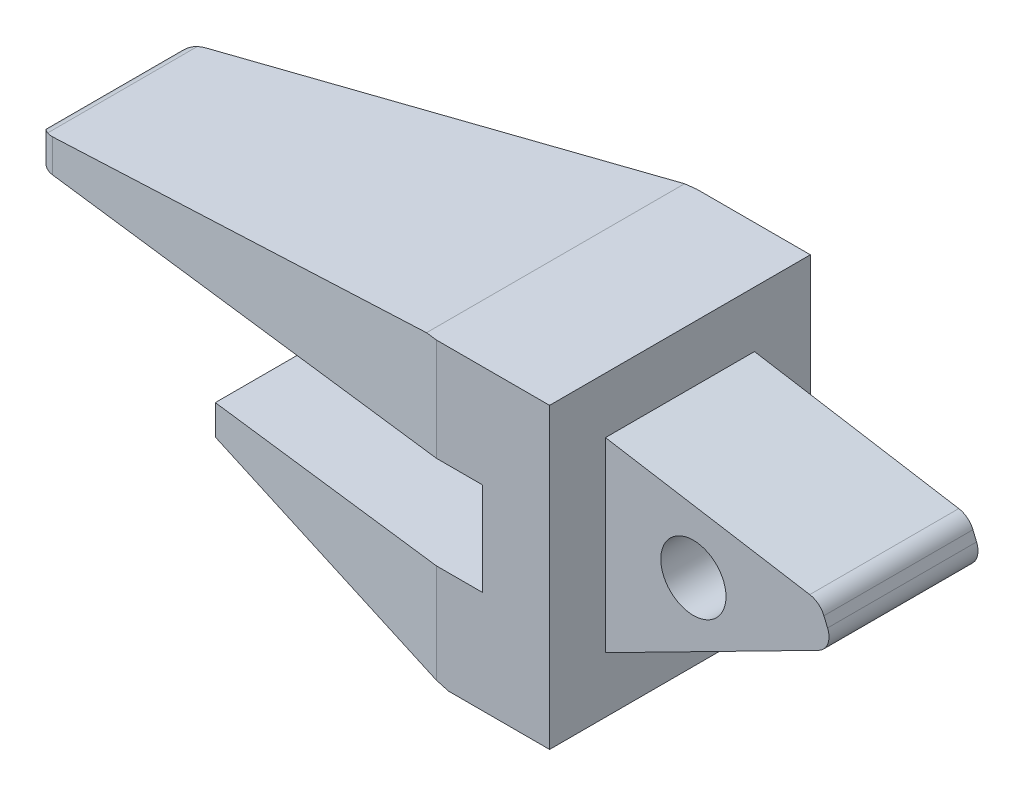
from build123d import *

# Parameters (mm, degrees)
BOSS_EXTRUDE1_DEPTH      = 80
CUT_EXTRUDE1_DEPTH       = 177.164695669
CUT_EXTRUDE1_DEPTH_BACK  = 177.164695669
SKETCH2_OUTSIDE_W        = 192.26
SKETCH2_OUTSIDE_H        = 119.26
BOSS_EXTRUDE2_DEPTH      = 20
BOSS_EXTRUDE2_DEPTH_BACK = 20
M20_TAPPED_HOLE1_D       = 17.5


with BuildPart() as part:
    # Sketch1 → Boss-Extrude1 (new body)
    with BuildSketch(Plane(origin=(0, 0, 0), x_dir=(1, 0, 0), z_dir=(0, 1, 0))):
        with BuildLine():
            Line((0, 14.689353522), (0, -14.689353522))
            ThreePointArc((0, -14.689353522), (1.507118597, -18.666037655), (5.271338899, -20.644943585))
            Line((5.271338899, -20.644943585), (122.6, -35))
            Line((122.6, -35), (153, -35))
            Line((153, -35), (153, 35))
            Line((153, 35), (122.6, 35))
            Line((122.6, 35), (5.271338899, 20.644943585))
            ThreePointArc((5.271338899, 20.644943585), (1.507118597, 18.666037655), (0, 14.689353522))
        make_face()
    extrude(amount=BOSS_EXTRUDE1_DEPTH)

    # Sketch2 outside → Cut-Extrude1 (cut, two sides: drawn at the far end of the back side and taken through both)
    with BuildSketch(Plane.XY.offset(-CUT_EXTRUDE1_DEPTH_BACK)):
        with Locations((76.5, 40)):
            Rectangle(SKETCH2_OUTSIDE_W, SKETCH2_OUTSIDE_H)
        with BuildLine():
            Line((153, 80), (153, 0))
            Line((153, 0), (125.9, 0))
            Line((125.9, 0), (55, 19.5))
            Line((55, 19.5), (55, 27.5))
            Line((55, 27.5), (135, 27.5))
            Line((135, 27.5), (135, 52.5))
            Line((135, 52.5), (0, 52.5))
            Line((0, 52.5), (0, 57.099356274))
            ThreePointArc((0, 57.099356274), (0.95248476, 59.69023467), (3.35632543, 61.047226972))
            Line((3.35632543, 61.047226972), (119.6, 80))
            Line((119.6, 80), (153, 80))
        make_face(mode=Mode.SUBTRACT)
    extrude(amount=CUT_EXTRUDE1_DEPTH + CUT_EXTRUDE1_DEPTH_BACK, mode=Mode.SUBTRACT)

    # Sketch3 → Boss-Extrude2 (add, two sides: drawn at the far end of the back side and taken through both)
    with BuildSketch(Plane.XY.offset(-BOSS_EXTRUDE2_DEPTH_BACK)):
        with BuildLine():
            Line((153, 65), (153, 15))
            Line((153, 15), (210.269952499, 44.180498289))
            ThreePointArc((210.269952499, 44.180498289), (212.69221031, 46.908347535), (212.616617933, 50.555645193))
            Line((212.616617933, 50.555645193), (211.637866551, 52.908901571))
            ThreePointArc((211.637866551, 52.908901571), (210.127565677, 54.906796263), (207.837878429, 55.921648096))
            Line((207.837878429, 55.921648096), (153, 65))
        make_face()
    extrude(amount=BOSS_EXTRUDE2_DEPTH + BOSS_EXTRUDE2_DEPTH_BACK)

    # M20 Tapped Hole1 (through all)
    with Locations(Plane.XY.offset(20)):
        with Locations((176.6, 44.2)):
            Hole(M20_TAPPED_HOLE1_D / 2)


solid = part.part
